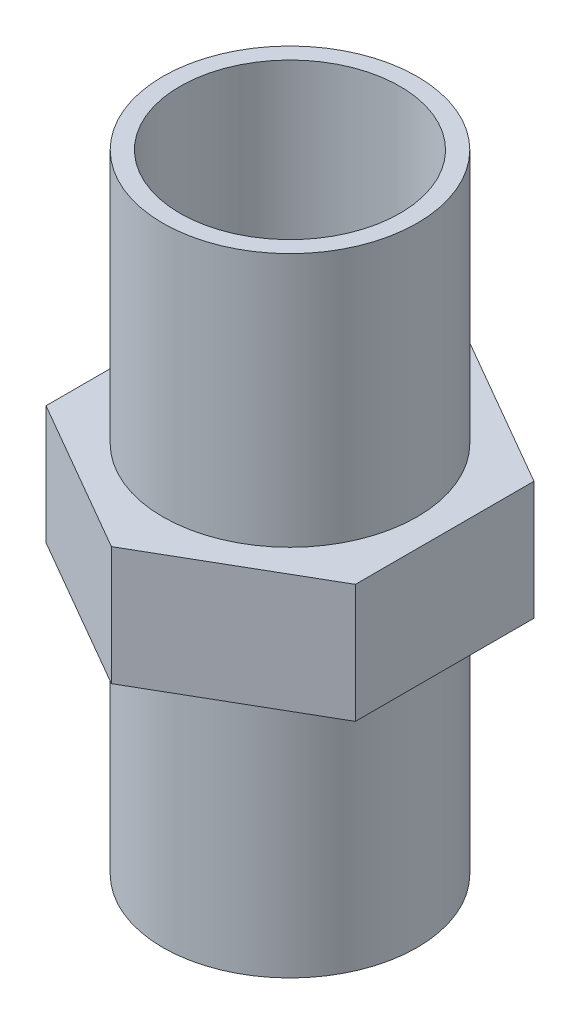
from build123d import *

# Parameters (mm, degrees)
SKETCH1_R           = 7.5
BOSS_EXTRUDE1_DEPTH = 15
BOSS_EXTRUDE2_DEPTH = 7
SKETCH3_R           = 7.5
BOSS_EXTRUDE3_DEPTH = 15
SKETCH4_R           = 6.489023352
CUT_EXTRUDE1_DEPTH  = 40.537347476


with BuildPart() as part:
    # Sketch1 → Boss-Extrude1 (new body)
    with BuildSketch(Plane(origin=(0, 0, 0), x_dir=(1, 0, 0), z_dir=(0, 1, 0))):
        with Locations(Location((0, 0, 0), (0, 0, 270))):
            Circle(SKETCH1_R)
    extrude(amount=BOSS_EXTRUDE1_DEPTH)

    # Sketch2 → Boss-Extrude2 (add)
    with BuildSketch(Plane(origin=(0, 15, 0), x_dir=(1, 0, 0), z_dir=(0, 1, 0))):
        Polygon((-9.123012787, 5.267173889), (-9.123012787, -5.267173889), (0, -10.534347777), (9.123012787, -5.267173889), (9.123012787, 5.267173889), (0, 10.534347777), align=None)
    extrude(amount=BOSS_EXTRUDE2_DEPTH)

    # Sketch3 → Boss-Extrude3 (add)
    with BuildSketch(Plane(origin=(0, 22, 0), x_dir=(1, 0, 0), z_dir=(0, 1, 0))):
        with Locations(Location((0, 0, 0), (0, 0, 270))):
            Circle(SKETCH3_R)
    extrude(amount=BOSS_EXTRUDE3_DEPTH)

    # Sketch4 → Cut-Extrude1 (cut, through all)
    with BuildSketch(Plane(origin=(0, 37, 0), x_dir=(1, 0, 0), z_dir=(0, 1, 0))):
        with Locations(Location((0, 0, 0), (0, 0, 270))):
            Circle(SKETCH4_R)
    extrude(amount=-CUT_EXTRUDE1_DEPTH, mode=Mode.SUBTRACT)


solid = part.part
